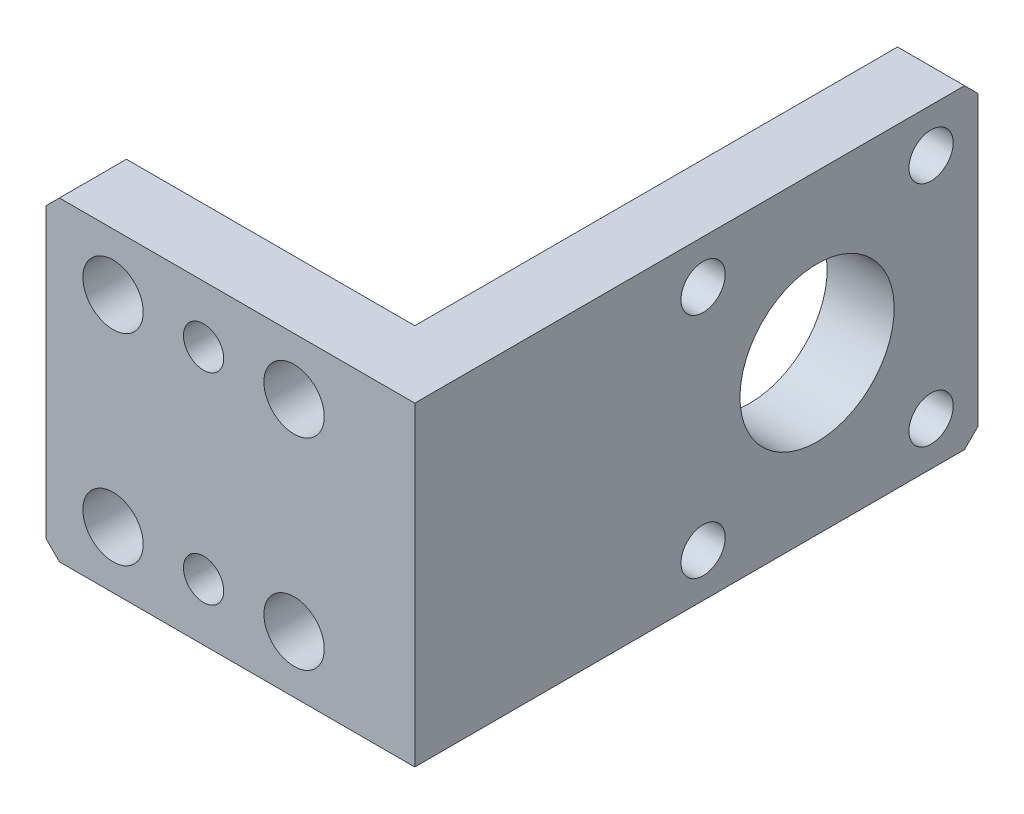
SolidWorks part; units mm, degrees
material "Q235-A"
ref_plane "Front Plane" through (0, 0, 0) normal (0, 0, 1) x (1, 0, 0)
ref_plane "Top Plane" through (0, 0, 0) normal (0, 1, 0) x (1, 0, 0)
ref_plane "Right Plane" through (0, 0, 0) normal (1, 0, 0) x (0, 0, -1)
sketch "Sketch1" plane through (0, 0, 0) normal (0, 0, 1) x (1, 0, 0)
  line L1 (-27.5, 23.5) -> (27.5, 23.5)
  line L2 (-27.5, 23.5) -> (-27.5, -23.5)
  line L3 (-27.5, -23.5) -> (27.5, -23.5)
  line L4 (27.5, 23.5) -> (27.5, -23.5)
  line L5 (-27.5, 23.5) -> (27.5, -23.5) construction
  line L6 (-27.5, -23.5) -> (27.5, 23.5) construction
  point P0 (0, 0)
  dimension "D1" = 55
  dimension "D2" = 47
extrude "Boss-Extrude1" add sketch "Sketch1" along normal blind 10
sketch "Sketch4" plane through (0, 0, 0) normal (0, 0, -1) x (-1, 0, 0)
  line L0 (-27.5, 23.5) -> (27.5, 23.5) construction
  line L1 (-17.5, 23.5) -> (-27.5, 23.5)
  line L2 (-17.5, 23.5) -> (-17.5, -23.5)
  line L3 (-17.5, -23.5) -> (-27.5, -23.5)
  line L4 (-27.5, 23.5) -> (-27.5, -23.5)
  line L5 (27.5, -23.5) -> (-27.5, -23.5) construction
  line L6 (-27.5, -23.5) -> (-27.5, 23.5) construction
  dimension "D1" = 10
extrude "Boss-Extrude2" add sketch "Sketch4" along normal blind 74
hole_wizard "M8 Clearance Hole1" positions "Sketch6" profile "Sketch7" hole size "M8" standard "GB"
sketch "Sketch6" plane through (0, 0, 0) normal (0, 0, -1) x (-1, 0, 0)
  line L0 (27.5, 0) -> (-40.8743, 0) construction
  line L1 (27.5, 23.5) -> (27.5, -23.5) construction
  line L3 (-17.5, -23.5) -> (-17.5, 23.5) construction
  point P0 (17.5, -15)
  point P2 (17.5, 15)
  point P4 (-9.5, -15)
  point P6 (-9.5, 15)
  dimension "D1" = 30
  dimension "D2" = 27
  dimension "D3" = 8
sketch "Sketch7" plane through (-17.5, -15, 0) normal (1, 0, 0) x (0, 1, 0)
  line L0 (0, 0) -> (0, 123.7039)
  line L1 (0, 123.7039) -> (4.5, 121)
  line L2 (4.5, 121) -> (4.5, 0)
  line L5 (4.5, 0) -> (0, 0)
  line L10 (0, 123.7039) -> (-4.5, 121) construction
  line L11 (0, -6.35) -> (0, 107.95) construction
  dimension "孔直径" = 9
  dimension "孔深度" = 121
  dimension "导头角度" = 118
chamfer "Chamfer1" distance 2 angle 45 2 edges at (-27.5, -23.5, 5) (-27.5, 23.5, 5)
sketch "Sketch8" plane through (17.5, 0, 0) normal (-1, 0, 0) x (0, 0, 1)
  line L0 (-74, 0) -> (27.7208, 0) construction
  line L1 (-74, -23.5) -> (-74, 23.5) construction
  line L2 (10, 21.5) -> (10, -21.5) construction
  circle A0 centre (-50, 0) radius 11.5
  dimension "D1" = 23
  dimension "D2" = 60
extrude "Cut-Extrude1" cut sketch "Sketch8" against normal blind 30
chamfer "Chamfer2" distance 2 angle 45 2 edges at (22.5, 23.5, -74) (22.5, -23.5, -74)
hole_wizard "Size mm blind dowel hole 1" positions "Sketch11" profile "Sketch12" hole size "Ø6.0" standard "GB" end condition through all
sketch "Sketch11" plane through (0, 0, 0) normal (0, 0, -1) x (-1, 0, 0)
  line L0 (-27.5, 0) -> (55.4, 0)
  line L1 (-27.5, 21.5) -> (-27.5, -21.5) construction
  line L4 (-9.5, 15) -> (17.5, 15)
  line L7 (-9.5, -15) -> (17.5, -15)
  line L10 (4, 15) -> (4, -15)
  point P0 (4, -15)
  point P2 (4, 15)
  dimension "D1" = 0
  dimension "D2" = 0
sketch "Sketch12" plane through (-4, -15, 0) normal (1, 0, 0) x (0, 1, 0)
  line L0 (0, 0) -> (0, 10)
  line L1 (0, 10) -> (3, 10)
  line L2 (3, 10) -> (3, 0)
  line L5 (3, 0) -> (0, 0)
  line L11 (0, -6.35) -> (0, 107.95) construction
  dimension "通孔孔直径" = 6
  dimension "通孔孔深度" = 10
hole_wizard "Hole size (per socket head cap screw type)1" positions "Sketch13" profile "Sketch14" counterbore size "M6" standard "GB"
sketch "Sketch13" plane through (17.5, 0, 0) normal (-1, 0, 0) x (0, 0, 1)
  circle A0 centre (-50, 0) radius 11.5 construction
  point P2 (-67, -17)
  dimension "D1" = 17
  dimension "D2" = 17
sketch "Sketch14" plane through (17.5, -17, -67) normal (0, 1, 0) x (0, 0, 1)
  line L0 (0, 0) -> (0, 34.7328)
  line L1 (0, 34.7328) -> (3.3, 32.75)
  line L2 (3.3, 32.75) -> (3.3, 5)
  line L3 (3.3, 5) -> (5.5, 5)
  line L4 (5.5, 5) -> (5.5, 0)
  line L5 (5.5, 0) -> (0, 0)
  line L10 (0, 34.7328) -> (-3.3, 32.75) construction
  line L11 (0, -6.35) -> (0, 107.95) construction
  dimension "孔直径" = 6.6
  dimension "孔深度" = 32.75
  dimension "柱形沉头孔直径" = 11
  dimension "柱形沉头孔深度" = 5
  dimension "导头角度" = 118
pattern_circular "CirPattern1" count 4 over 360 about axis through (0, 0, -50) along (1, 0, 0) of "Hole size (per socket head cap screw type)1"
